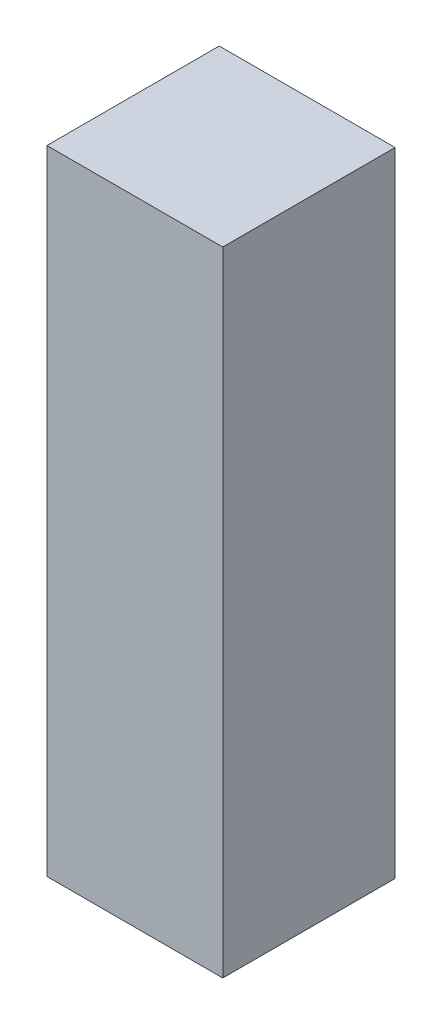
from build123d import *

# Parameters (mm, degrees)
SKETCH_1_W      = 25
SKETCH_1_H      = 90
EXTRUDE_1_DEPTH = 24.5


with BuildPart() as part:
    # 草图1 → 凸台-拉伸1 (new body)
    with BuildSketch(Plane.XY):
        with Locations((12.5, 0)):
            Rectangle(SKETCH_1_W, SKETCH_1_H)
    extrude(amount=EXTRUDE_1_DEPTH)


solid = part.part
